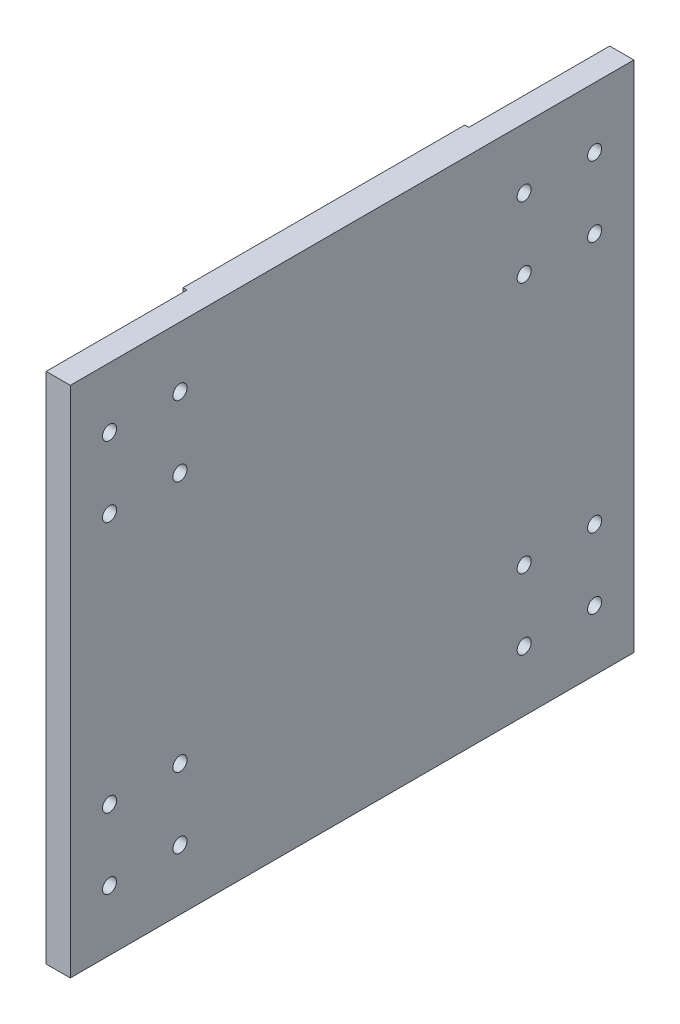
SolidWorks part; units mm, degrees
other "Annotation1"
sketch "草图4" plane through (0, -160, -150) normal (-0.5532, -0.1245, -0.8237) x (-0.6996, -0.4675, 0.5405)
material "普通碳钢"
ref_plane "Front Plane" through (0, 0, 0) normal (0, 0, 1) x (1, 0, 0)
ref_plane "Top Plane" through (0, 0, 0) normal (0, 1, 0) x (1, 0, 0)
ref_plane "Right Plane" through (0, 0, 0) normal (1, 0, 0) x (0, 0, -1)
sketch "Sketch1" plane through (0, 0, 0) normal (1, 0, 0) x (0, 0, -1)
  line L0 (-85.5, 97.5) -> (85.5, 97.5) construction
  line L1 (-140, -127.5) -> (140, -127.5)
  line L2 (-140, -127.5) -> (-140, 127.5)
  line L3 (-140, 127.5) -> (140, 127.5)
  line L4 (140, -127.5) -> (140, 127.5)
  line L5 (-140, -127.5) -> (140, 127.5) construction
  line L6 (-140, 127.5) -> (140, -127.5) construction
  line L7 (0, 97.5) -> (0, 127.5) construction
  circle A0 centre (-120.5, 97.5) radius 3.5
  circle A1 centre (-85.5, 97.5) radius 3.5
  circle A2 centre (-120.5, -97.5) radius 3.5
  circle A3 centre (-85.5, -97.5) radius 3.5
  circle A4 centre (-120.5, 62.5) radius 3.5
  circle A5 centre (-85.5, 62.5) radius 3.5
  circle A6 centre (-120.5, -62.5) radius 3.5
  circle A7 centre (-85.5, -62.5) radius 3.5
  circle A8 centre (85.5, 97.5) radius 3.5
  circle A9 centre (120.5, 97.5) radius 3.5
  circle A10 centre (85.5, -62.5) radius 3.5
  circle A11 centre (120.5, -62.5) radius 3.5
  circle A12 centre (85.5, -97.5) radius 3.5
  circle A13 centre (120.5, -97.5) radius 3.5
  circle A14 centre (85.5, 62.5) radius 3.5
  circle A15 centre (120.5, 62.5) radius 3.5
  point P0 (0, 0)
  dimension "D3" = 7
  dimension "D1" = 255
  dimension "D2" = 280
  dimension "D4" = 35
  dimension "D5" = 35
  dimension "D6" = 206
  dimension "D8" = 30
  dimension "D9" = 35
  dimension "D10" = 160
  dimension "D11" = 35
extrude "Boss-Extrude1" add sketch "Sketch1" along normal blind 14
sketch "Sketch2" plane through (0, 127.5, 0) normal (0, 1, 0) x (1, 0, 0)
  line L0 (0, 140) -> (0, -140) construction
  line L1 (0, 140) -> (2, 140)
  line L2 (0, 140) -> (0, 60)
  line L3 (0, 60) -> (2, 60)
  line L4 (2, 140) -> (2, 60)
  line L5 (0, 140) -> (2, 60) construction
  line L6 (0, 60) -> (2, 140) construction
  line L12 (0, 0) -> (14, 0) construction
  line L13 (14, 140) -> (14, -140) construction
  line L14 (0, -60) -> (2, -60)
  line L15 (2, -140) -> (2, -60)
  line L16 (0, -140) -> (2, -140)
  line L17 (0, -140) -> (0, -60)
  line L18 (14, 140) -> (0, 140) construction
  point P4 (1, 100)
  dimension "D2" = 80
  dimension "D3" = 2
sketch "Sketch3" plane through (0, -127.5, 0) normal (0, -1, 0) x (1, 0, 0)
  line L1 (0, -140) -> (3.8417, -140)
  line L2 (0, -140) -> (0, -60)
  line L3 (0, -60) -> (3.8417, -60)
  line L4 (3.8417, -140) -> (3.8417, -60)
  line L5 (0, -140) -> (3.8417, -60) construction
  line L6 (0, -60) -> (3.8417, -140) construction
  line L7 (0, 140) -> (2, 140)
  line L8 (0, 140) -> (0, 60)
  line L9 (0, 60) -> (2, 60)
  line L10 (2, 140) -> (2, 60)
  line L11 (0, 140) -> (2, 60) construction
  line L12 (0, 60) -> (2, 140) construction
  point P4 (1.9209, -100)
  point P10 (1, 100)
  dimension "D1" = 80
  dimension "D2" = 80
  dimension "D3" = 2
sketch "Sketch6" plane through (0, 0, 0) normal (-1, 0, 0) x (0, 0, 1)
  line L0 (140, -127.5) -> (-140, -127.5) construction
  line L1 (-140, 127.5) -> (-70, 127.5)
  line L2 (-140, 127.5) -> (-140, -127.5)
  line L3 (-140, -127.5) -> (-70, -127.5)
  line L4 (-70, 127.5) -> (-70, -127.5)
  line L5 (0, 127.5) -> (0, 140.4174) construction
  line L6 (-140, 127.5) -> (140, 127.5) construction
  line L7 (70, 127.5) -> (70, -127.5)
  line L8 (140, -127.5) -> (70, -127.5)
  line L9 (140, 127.5) -> (140, -127.5)
  line L10 (140, 127.5) -> (70, 127.5)
  dimension "D1" = 70
extrude "Cut-Extrude3" cut sketch "Sketch6" against normal blind 2
